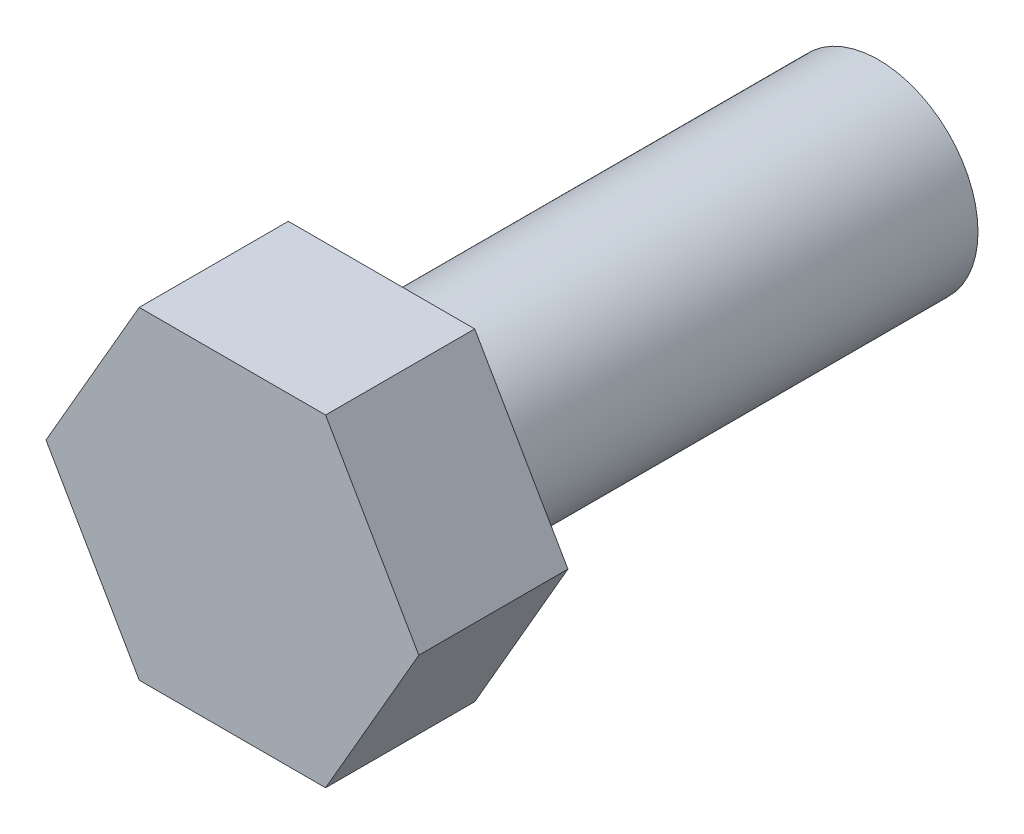
SolidWorks part; units mm, degrees
ref_plane "Front Plane" through (0, 0, 0) normal (0, 0, 1) x (1, 0, 0)
ref_plane "Top Plane" through (0, 0, 0) normal (0, 1, 0) x (1, 0, 0)
ref_plane "Right Plane" through (0, 0, 0) normal (1, 0, 0) x (0, 0, -1)
sketch "Sketch1" plane through (0, 0, 0) normal (0, 0, 1) x (1, 0, 0)
  circle A0 centre (0, 0) radius 4
  dimension "D1" = 8
extrude "Boss-Extrude1" add sketch "Sketch1" along normal blind 20
sketch "Sketch2" plane through (0, 0, 20) normal (0, 0, 1) x (1, 0, 0)
  line L1 (-3.75, 6.4952) -> (-7.5, 0)
  line L2 (-7.5, 0) -> (-3.75, -6.4952)
  line L3 (-3.75, -6.4952) -> (3.75, -6.4952)
  line L4 (3.75, -6.4952) -> (7.5, 0)
  line L5 (7.5, 0) -> (3.75, 6.4952)
  line L6 (3.75, 6.4952) -> (-3.75, 6.4952)
  circle A0 centre (0, 0) radius 6.4952 construction
  dimension "D1" = 15
extrude "Boss-Extrude2" add sketch "Sketch2" along normal blind 6
